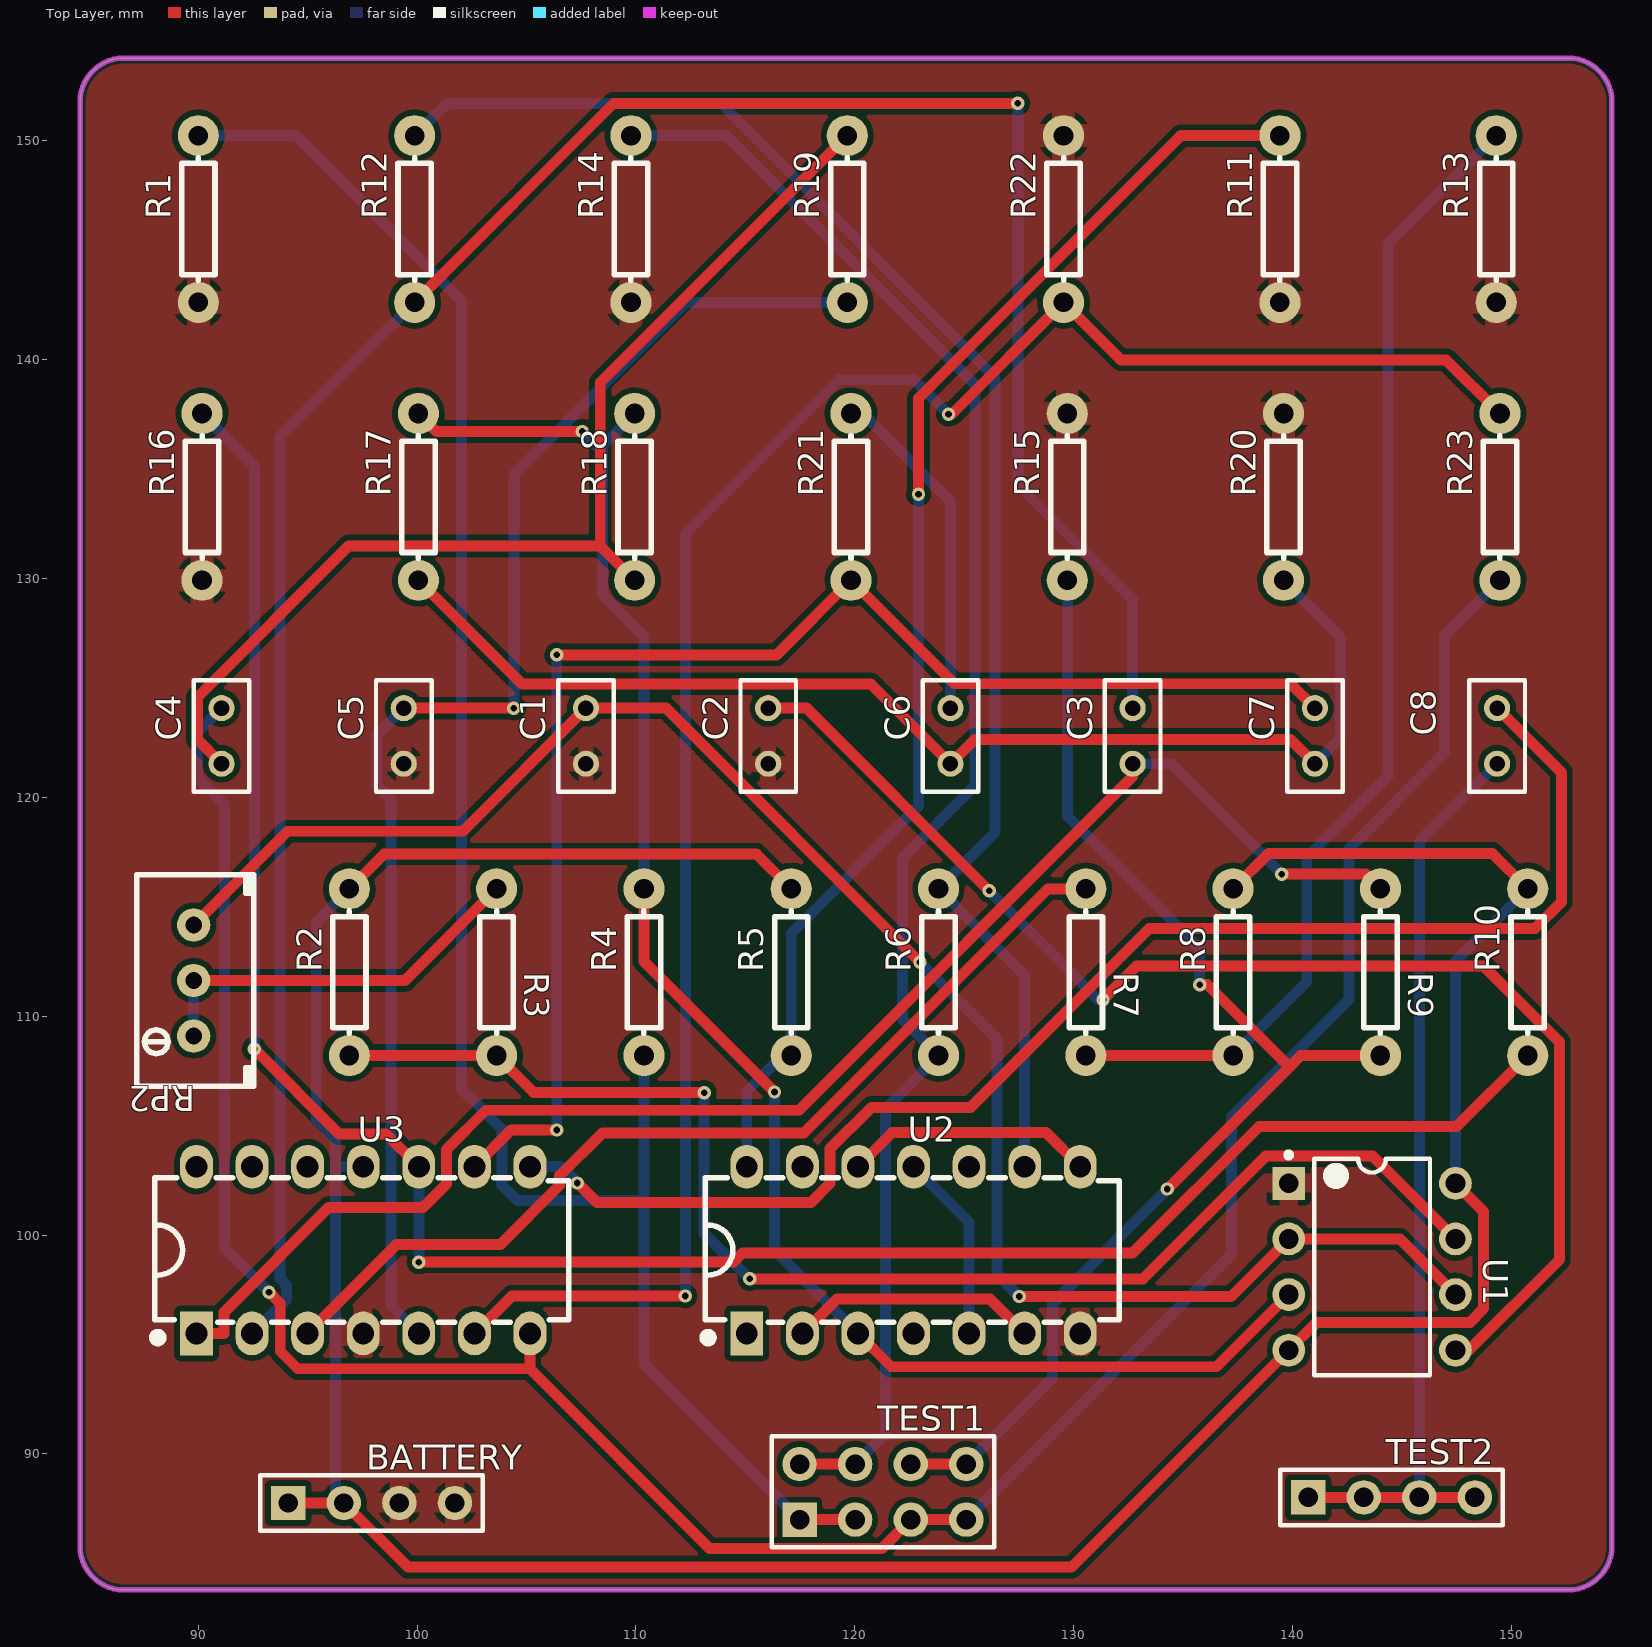
[diagram p0: Top Layer view]
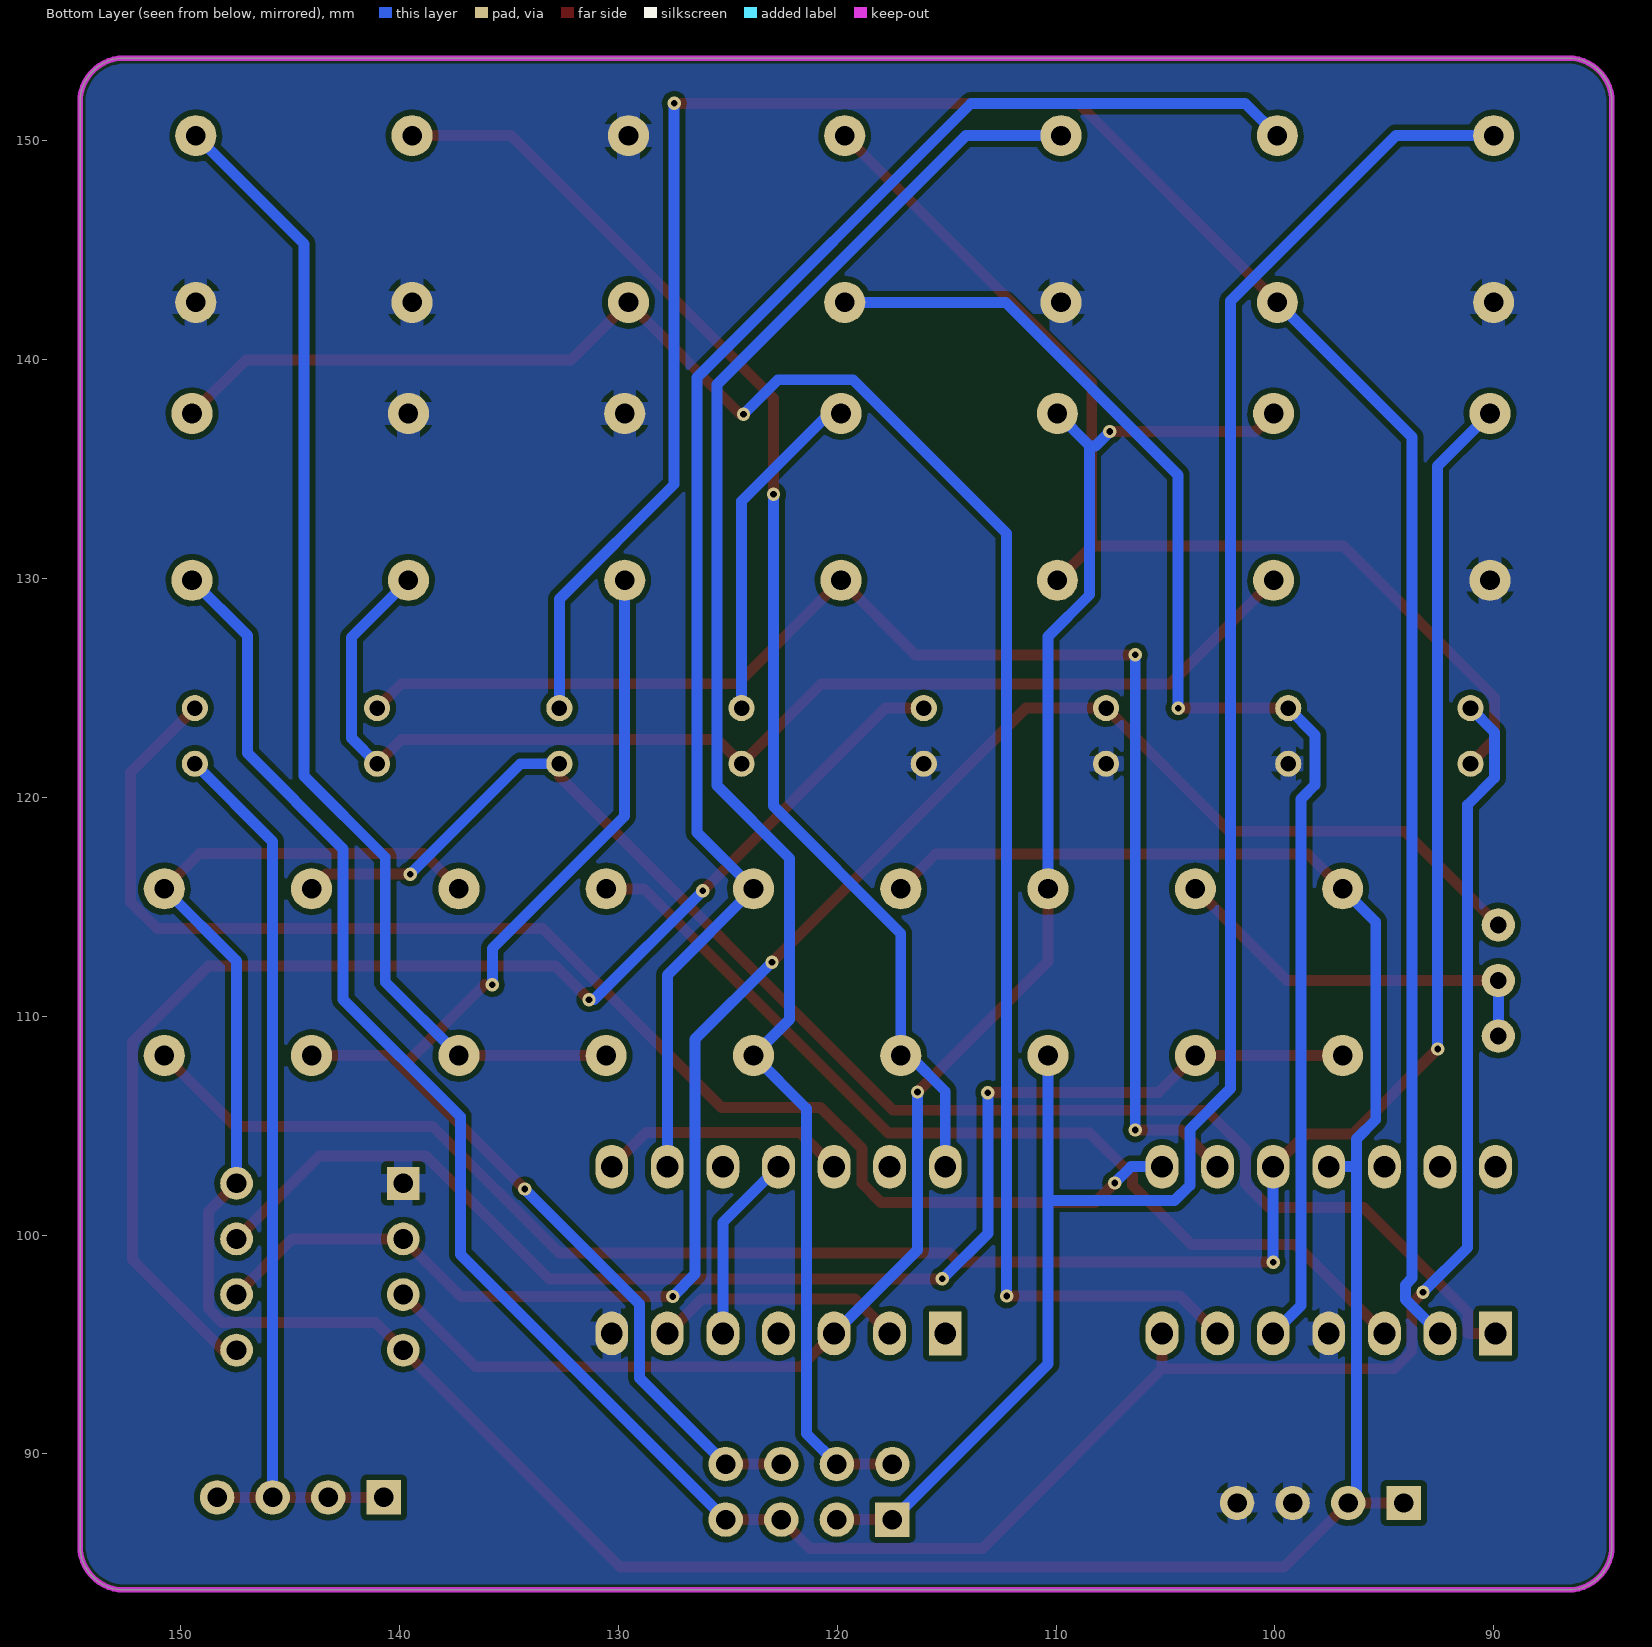
[diagram p1: Bottom Layer view, seen from below]
# Altium PCB MISC51938.pcbdoc
Units mm, origin at the board's own origin, x right, y up, seen from the top; angles counter-clockwise.
Board outline 70 x 70 mm, 2 copper layers (Top Layer, Bottom Layer), stack 0 mm thick; 38 components, 29 nets, 117 pads, 22 vias.

## Layer stack, top to bottom
Top Layer: signal copper (thickness not stored)
Bottom Layer: signal copper (thickness not stored)

## Board outline
84.597,151.785 cw(c86.597,151.785) 86.597,153.785 152.597,153.785 cw(c152.597,151.785) 154.597,151.785 154.597,85.785 cw(c152.597,85.785) 152.597,83.785 86.597,83.785 cw(c86.597,85.785) 84.597,85.785 84.597,151.785

## Design rules (kind name [scope] priority, off if disabled: settings)
BoardOutlineClearance Plane_Default_1 [All] p2 off: genericclearance=0.25 ignorepadtopadclearanceinfootprint=FALSE except(0: Arc-SplitContinuation Track-SplitContinuation SMDPad-SplitContinuation THPad-SplitContinuation Via-SplitContinuation Fill-SplitContinuation Region-SplitContinuation Poly-SplitContinuation Text-SplitContinuation Hole-SplitContinuation; 0.25: Arc-OutlineEdge Track-OutlineEdge SMDPad-OutlineEdge THPad-OutlineEdge Via-OutlineEdge Fill-OutlineEdge Region-OutlineEdge Poly-OutlineEdge Text-OutlineEdge Hole-OutlineEdge Arc-CutoutEdge Track-CutoutEdge SMDPad-CutoutEdge THPad-CutoutEdge Via-CutoutEdge Fill-CutoutEdge Region-CutoutEdge Poly-CutoutEdge Text-CutoutEdge Hole-CutoutEdge)
BoardOutlineClearance Copper_Default_1 [All] p4 off: genericclearance=0.25 ignorepadtopadclearanceinfootprint=FALSE except(0: Arc-SplitContinuation Track-SplitContinuation SMDPad-SplitContinuation THPad-SplitContinuation Via-SplitContinuation Fill-SplitContinuation Region-SplitContinuation Poly-SplitContinuation Text-SplitContinuation Hole-SplitContinuation; 0.25: Arc-OutlineEdge Track-OutlineEdge SMDPad-OutlineEdge THPad-OutlineEdge Via-OutlineEdge Fill-OutlineEdge Region-OutlineEdge Poly-OutlineEdge Text-OutlineEdge Hole-OutlineEdge Arc-CutoutEdge Track-CutoutEdge SMDPad-CutoutEdge THPad-CutoutEdge Via-CutoutEdge Fill-CutoutEdge Region-CutoutEdge Poly-CutoutEdge Text-CutoutEdge Hole-CutoutEdge)
BoardOutlineClearance Copper_gge9694_1 [All] p6 off: genericclearance=0.25 ignorepadtopadclearanceinfootprint=FALSE except(0: Arc-SplitContinuation Track-SplitContinuation SMDPad-SplitContinuation THPad-SplitContinuation Via-SplitContinuation Fill-SplitContinuation Region-SplitContinuation Poly-SplitContinuation Text-SplitContinuation Hole-SplitContinuation; 0.25: Arc-OutlineEdge Track-OutlineEdge SMDPad-OutlineEdge THPad-OutlineEdge Via-OutlineEdge Fill-OutlineEdge Region-OutlineEdge Text-OutlineEdge Hole-OutlineEdge Arc-CutoutEdge Track-CutoutEdge SMDPad-CutoutEdge THPad-CutoutEdge Via-CutoutEdge Fill-CutoutEdge Region-CutoutEdge Text-CutoutEdge Hole-CutoutEdge; 0.254: Poly-OutlineEdge Poly-CutoutEdge)
BoardOutlineClearance Copper_gge9712_1 [All] p8 off: genericclearance=0.25 ignorepadtopadclearanceinfootprint=FALSE except(0: Arc-SplitContinuation Track-SplitContinuation SMDPad-SplitContinuation THPad-SplitContinuation Via-SplitContinuation Fill-SplitContinuation Region-SplitContinuation Poly-SplitContinuation Text-SplitContinuation Hole-SplitContinuation; 0.25: Arc-OutlineEdge Track-OutlineEdge SMDPad-OutlineEdge THPad-OutlineEdge Via-OutlineEdge Fill-OutlineEdge Region-OutlineEdge Text-OutlineEdge Hole-OutlineEdge Arc-CutoutEdge Track-CutoutEdge SMDPad-CutoutEdge THPad-CutoutEdge Via-CutoutEdge Fill-CutoutEdge Region-CutoutEdge Text-CutoutEdge Hole-CutoutEdge; 0.254: Poly-OutlineEdge Poly-CutoutEdge)
BoardOutlineClearance Default_1 [All] p10: genericclearance=0.25 ignorepadtopadclearanceinfootprint=FALSE except(0: Arc-SplitContinuation Track-SplitContinuation SMDPad-SplitContinuation THPad-SplitContinuation Via-SplitContinuation Fill-SplitContinuation Region-SplitContinuation Poly-SplitContinuation Text-SplitContinuation Hole-SplitContinuation; 0.25: Arc-OutlineEdge Track-OutlineEdge SMDPad-OutlineEdge THPad-OutlineEdge Via-OutlineEdge Fill-OutlineEdge Region-OutlineEdge Poly-OutlineEdge Text-OutlineEdge Hole-OutlineEdge Arc-CutoutEdge Track-CutoutEdge SMDPad-CutoutEdge THPad-CutoutEdge Via-CutoutEdge Fill-CutoutEdge Region-CutoutEdge Poly-CutoutEdge Text-CutoutEdge Hole-CutoutEdge)
Clearance Plane_Default [All] p1 off: gap=0.25 ignorepadtopadclearanceinfootprint=FALSE
Clearance Copper_Default [All] p3 off: gap=0.25 ignorepadtopadclearanceinfootprint=FALSE
Clearance Copper_gge9694 [All] p5 off: gap=0.25 ignorepadtopadclearanceinfootprint=FALSE except(0.254: Poly-Track Poly-SMDPad Poly-THPad Poly-Via Poly-Fill Poly-Region Poly-Poly Poly-Arc Poly-Text Poly-Hole)
Clearance Copper_gge9712 [All] p7 off: gap=0.25 ignorepadtopadclearanceinfootprint=FALSE except(0.254: Poly-Track Poly-SMDPad Poly-THPad Poly-Via Poly-Fill Poly-Region Poly-Poly Poly-Arc Poly-Text Poly-Hole)
Clearance Default [All] p9: gap=0.25 ignorepadtopadclearanceinfootprint=FALSE
PasteMaskExpansion Common [All] p1: expansion=0
PlaneConnect Default_4 [All] p1: planeconnectstyle=Relief reliefexpansion=0.508 reliefentries=4 reliefconductorwidth=0 reliefairgap=0.254
PolygonConnect gge9694 [All] p1 off: connectstyle=Relief reliefconductorwidth=0 reliefentries=4 polygonreliefangle="90 Angle" airgapwidth=0.254 via.connectstyle=Relief via.reliefconductorwidth=0.254 via.reliefentries=4 via.polygonreliefangle="90 Angle" via.airgapwidth=0.254
PolygonConnect gge9712 [All] p2 off: connectstyle=Relief reliefconductorwidth=0 reliefentries=4 polygonreliefangle="90 Angle" airgapwidth=0.254 via.connectstyle=Relief via.reliefconductorwidth=0.254 via.reliefentries=4 via.polygonreliefangle="90 Angle" via.airgapwidth=0.254
PolygonConnect Default_5 [All] p3: connectstyle=Relief reliefconductorwidth=0 reliefentries=4 polygonreliefangle="90 Angle" airgapwidth=0.254 via.connectstyle=Relief via.reliefconductorwidth=0.254 via.reliefentries=4 via.polygonreliefangle="90 Angle" via.airgapwidth=0.254
RoutingVias Default_3 [All] p1: holewidth=0.305 width=0.61 viastyle="Through Hole" minholewidth=0.305 minwidth=0.61 maxholewidth=59.995 maxwidth=100.025
SolderMaskExpansion Common_1 [IsVia] p1: expansion=-25.4 istentingtop=TRUE
SolderMaskExpansion Common_1 [All] p2: expansion=0.051 istentingtop=FALSE
Width Default_2 [All] p1: maxlimit=25.4 minlimit=0.5 preferedwidth=0.5

## Components (designator, comment, footprint, x,y, rotation, side; value= is the part's Value field where it differs from the comment)
BATTERY "HDR-M-2.54_1x4" HDR-M-2.54_1X4 97.917,87.757 r0 top
C1 "1n" RAD-0.1 107.714,122.809 r90 top
C2 "0.01u" RAD-0.1 116.042,122.809 r90 top
C3 "10n" RAD-0.1 132.697,122.809 r90 top
C4 "1n" RAD-0.1 91.059,122.809 r90 top
C5 "1n" RAD-0.1 99.387,122.809 r90 top
C6 "0.1n" RAD-0.1 124.369,122.809 r90 top
C7 "0.1n" RAD-0.1 141.024,122.809 r90 top
C8 "1n" RAD-0.1 149.352,122.809 r90 top
R1 "60" R_AXIAL-0.3 90.001,146.431 r90 top
R2 "510" R_AXIAL-0.3 96.901,112.014 r90 top
R3 "12k" R_AXIAL-0.3 103.632,112.014 r270 top
R4 "540" R_AXIAL-0.3 110.363,112.014 r90 top
R5 "1k" R_AXIAL-0.3 117.094,112.014 r90 top
R6 "480" R_AXIAL-0.3 123.825,112.014 r90 top
R7 "1k" R_AXIAL-0.3 130.556,112.014 r270 top
R8 "300" R_AXIAL-0.3 137.287,112.014 r90 top
R9 "400" R_AXIAL-0.3 144.018,112.014 r270 top
R10 "1k" R_AXIAL-0.3 150.749,112.014 r90 top
R11 "1k" R_AXIAL-0.3 139.425,146.431 r90 top
R12 "1800" R_AXIAL-0.3 99.885,146.431 r90 top
R13 "100" R_AXIAL-0.3 149.31,146.431 r90 top
R14 "120" R_AXIAL-0.3 109.77,146.431 r90 top
R15 "200" R_AXIAL-0.3 129.709,133.731 r90 top
R16 "1350" R_AXIAL-0.3 90.17,133.731 r90 top
R17 "41k" R_AXIAL-0.3 100.055,133.731 r90 top
R18 "10k" R_AXIAL-0.3 109.94,133.731 r90 top
R19 "16500" R_AXIAL-0.3 119.655,146.431 r90 top
R20 "50" R_AXIAL-0.3 139.594,133.731 r90 top
R21 "90k" R_AXIAL-0.3 119.825,133.731 r90 top
R22 "3600" R_AXIAL-0.3 129.54,146.431 r90 top
R23 "720" R_AXIAL-0.3 149.479,133.731 r90 top
RP2 "R_3296W_US" RES-ADJ-TH_3296W 89.789,111.633 r180 top
TEST1 "test" HDR-M-2.54_2X4 121.285,88.265 r0 top
TEST2 "test" HDR-M-2.54_1X4 144.526,88.011 r0 top
U1 "100kHz" DIP-8_L9.8-W6.6-P2.54-LS7.6-BL 143.637,98.552 r270 top
U2 "SN74LS74N" DIP-14_L19.1-W6.4-P2.54-LS7.6-BL 122.682,99.314 r0 top
U3 "LM324_C5157701" DIP-14_L18.9-W6.4-P2.54-LS7.6-BL 97.536,99.314 r0 top

## Footprints (in the part's own frame and the unit in brackets; to place one, negate y for a bottom-side part, rotate by r counter-clockwise, add the part's x,y. Pads: shape width x height; smd on the part's side, far side on the other; paste and mask are expansions set on the pad)
DIP-8_L9.8-W6.6-P2.54-LS7.6-BL [mm]
  rect 1.5x1.5 hole 0.9: 1(-3.81,-3.81)
  round 1.5 hole 0.9: 2(-1.27,-3.81) 3(1.27,-3.81) 4(3.81,-3.81) 5(3.81,3.81) 6(1.27,3.81) 7(-1.27,3.81) 8(-3.81,3.81)
  silkscreen extent -5.23,-3.93 4.96,2.65
DIP-14_L18.9-W6.4-P2.54-LS7.6-BL [mm]
  rect 1.5x2 hole 1: 1(-7.62,-3.81)
  oval 1.5x2 hole 1: 2(-5.08,-3.81) 3(-2.54,-3.81) 4(0,-3.81) 5(2.54,-3.81) 6(5.08,-3.81) 7(7.62,-3.81) 8(7.62,3.81) 9(5.08,3.81) 10(2.54,3.81) 11(0,3.81) 12(-2.54,3.81) 13(-5.08,3.81) 14(-7.62,3.81)
  silkscreen extent -9.59,-4.2 9.4,3.3
DIP-14_L19.1-W6.4-P2.54-LS7.6-BL [mm]
  rect 1.5x2 hole 1: 1(-7.62,-3.81)
  oval 1.5x2 hole 1: 2(-5.08,-3.81) 3(-2.54,-3.81) 4(0,-3.81) 5(2.54,-3.81) 6(5.08,-3.81) 7(7.62,-3.81) 8(7.62,3.81) 9(5.08,3.81) 10(2.54,3.81) 11(0,3.81) 12(-2.54,3.81) 13(-5.08,3.81) 14(-7.62,3.81)
  silkscreen extent -9.59,-4.2 9.4,3.3
HDR-M-2.54_1X4 [mil]
  rect 62x62 hole 35: 1(-150,0)
  round 62 hole 35: 2(-50,0) 3(50,0) 4(150,0)
  silkscreen extent -200,-50 200,50
HDR-M-2.54_2X4 [mil]
  rect 62x62 hole 35: 1(-150,-50)
  round 62 hole 35: 2(-150,50) 3(-50,-50) 4(-50,50) 5(50,-50) 6(50,50) 7(150,-50) 8(150,50)
  silkscreen extent -200,-100 200,100
R_AXIAL-0.3 [mil]
  round 74 hole 35.4: 1(-150,0) 2(150,0)
  silkscreen extent -110,-30 110,30
RAD-0.1 [mil]
  round 47 hole 28: 1(-50,0) 2(50,0)
  silkscreen extent -100,-50 100,50
RES-ADJ-TH_3296W [mil]
  round 60 hole 30 copper offset -0.01,0.01: 1(0.01,99.99) 2(0.01,-0.01) 3(0.01,-100.01)
  silkscreen extent -108,-190 102,190

## Via types
v1: diameter 0.61, hole 0.305, Top Layer to Bottom Layer, 22 vias

## Nets (pads, with @x,y where several pads share a name; then routed paths per layer and width w, separated by ;. In a path a pad name is that pad's centre, name@x,y a point inside that pad or via, vN(x,y) a via of type N, cw(c..) or ccw(c..) an arc to the next point about the centre after c; other vN are vias at no path point)
C4_1: C4.1 R18.1 R19.2 | length 50.4
  Top Layer w0.5: C4.1 89.954,122.644 89.954,124.577 96.87,131.493 108.368,131.493 ; R18.1 108.368,131.493 ; R19.2 108.368,138.953 108.368,131.493
C5_2: C5.2 R19.1 U3.5 | length 64.1
  Top Layer w0.5: C5.2 v1(104.419,124.079)
  Bottom Layer w0.5: C5.2 98.161,122.853 98.161,120.577 98.806,119.931 98.806,96.774 U3.5 ; v1(104.419,124.079) 104.419,134.741 112.299,142.621 R19.1
C6_1: C6.1 C7.1 R17.1 R20.1 | length 55.3
  Top Layer w0.5: R17.1 104.798,125.178 120.731,125.178 C6.1 125.482,122.651 139.912,122.651 C7.1
  Bottom Layer w0.5: R20.1 142.199,127.316 142.199,122.713 C7.1
C6_2: C6.2 R21.2 | length 15.7
  Bottom Layer w0.5: R21.2 120.363,137.541 124.369,133.534 C6.2
C7_2: C7.2 R21.1 U3.9 | length 64.6
  Top Layer w0.5: U3.9 104.296,104.804 v1(106.378,104.804) ; v1(106.378,126.515) 116.418,126.515 R21.1 124.552,125.194 139.91,125.194 C7.2
  Bottom Layer w0.5: v1(106.378,104.804) v1(106.378,126.515)
C8_1: C8.1 TEST2.1 TEST2.2 TEST2.3 TEST2.4 | length 42.6
  Top Layer w0.5: TEST2.1 TEST2.2 TEST2.3 TEST2.4
  Bottom Layer w0.5: TEST2.3 145.796,117.983 C8.1
GND: BATTERY.3 BATTERY.4 C1.1 C2.1 C5.1 R1.1 R11.1 R13.1 R14.1 R15.2 R16.1 R20.2 R22.2 U1.1 U2.7 U3.4
R3_1: R3.1 RP2.1 RP2.2 | length 18.1
  Top Layer w0.5: RP2.2 99.441,111.633 R3.1
  Bottom Layer w0.5: RP2.1 RP2.2
R4_1: R1.2 R4.1 TEST1.1 TEST1.3 | length 89.8
  Top Layer w0.5: TEST1.1 TEST1.3
  Bottom Layer w0.5: R1.2 94.461,150.241 102.021,142.681 102.021,106.696 103.887,104.83 103.887,102.263 104.579,101.572 110.363,101.572 ; R4.1 110.363,101.572 ; TEST1.1 110.363,94.107 110.363,101.572
R7_1: R7.1 U3.3 | length 44.2
  Top Layer w0.5: U3.3 99.062,99.569 103.804,99.569 106.512,102.277 106.512,102.712 108.469,104.669 117.665,104.669 128.82,115.824 R7.1
R7_2: R7.2 R8.1 R13.2 | length 53.7
  Top Layer w0.5: R7.2 R8.1
  Bottom Layer w0.5: R8.1 140.653,111.57 140.653,117.266 144.368,120.98 144.368,145.299 R13.2
R10_1: R10.1 R16.2 U3.10 | length 98.7
  Top Layer w0.5: v1(92.558,108.504) 96.437,104.626 98.574,104.626 U3.10 ; v1(100.076,98.763) 114.447,98.763 114.858,99.174 132.694,99.174 138.479,104.958 147.503,104.958 R10.1
  Bottom Layer w0.5: R16.2 92.558,135.153 v1(92.558,108.504) ; v1(100.076,98.763) U3.10
TEST1_2: R6.1 R14.2 TEST1.2 TEST1.4 | length 75.9
  Top Layer w0.5: TEST1.2 TEST1.4
  Bottom Layer w0.5: R14.2 114.117,150.241 125.496,138.862 125.496,120.542 122.172,117.218 122.172,109.857 R6.1 121.412,105.791 121.412,90.932 TEST1.4
TEST1_5: C4.2 R23.1 TEST1.5 TEST1.7 U3.7 | length 121.7
  Top Layer w0.5: v1(93.228,97.39) 93.744,96.874 93.744,94.691 94.544,93.891 105.156,93.891 ; U3.7 105.156,93.891 ; TEST1.7 TEST1.5 121.242,85.682 113.366,85.682 105.156,93.891
  Bottom Layer w0.5: C4.2 89.956,122.976 89.956,120.896 91.186,119.665 91.186,99.432 v1(93.228,97.39) ; TEST1.7 137.22,99.12 137.22,105.407 142.576,110.764 142.576,117.649 146.952,122.025 146.952,127.394 R23.1
TEST1_6: R9.2 R15.1 TEST1.6 TEST1.8 | length 57.8
  Top Layer w0.5: TEST1.6 TEST1.8 ; v1(134.282,102.108) 139.861,107.687 ; v1(135.758,111.442) 136.106,111.442 139.861,107.687 ; R9.2 140.378,108.204 139.861,107.687
  Bottom Layer w0.5: TEST1.8 129.032,93.472 129.032,96.858 v1(134.282,102.108) ; R15.1 129.709,119.154 135.758,113.105 v1(135.758,111.442)
U1_2: C1.2 RP2.3 U1.2 U1.6 | length 81.3
  Top Layer w0.5: RP2.3 94.07,118.455 102.09,118.455 C1.2 111.369,124.079 v1(122.979,112.469) ; v1(127.51,97.195) 137.2,97.195 U1.2 144.907,99.822 U1.6
  Bottom Layer w0.5: v1(122.979,112.469) 126.492,108.956 126.492,98.213 v1(127.51,97.195)
U1_3: R4.2 R17.2 R18.2 U1.3 U2.3 | length 78.2
  Top Layer w0.5: R17.2 100.874,136.722 v1(107.54,136.722) ; R4.2 110.363,112.51 v1(116.332,106.541) ; U2.3 121.664,93.982 136.527,93.982 U1.3
  Bottom Layer w0.5: v1(107.54,136.722) 108.201,136.062 108.46,136.062 ; R18.2 108.46,136.062 ; R4.2 110.363,127.36 108.46,129.263 108.46,136.062 ; v1(116.332,106.541) 116.332,99.314 U2.3
U1_5: C2.2 U1.5 | length 60.2
  Top Layer w0.5: C2.2 117.796,124.079 v1(126.146,115.729) ; v1(131.343,110.76) 132.877,112.294 148.725,112.294 152.195,108.825 152.195,98.875 148.062,94.742 U1.5
  Bottom Layer w0.5: v1(126.146,115.729) 131.115,110.76 v1(131.343,110.76)
U1_7: R2.1 R3.2 U1.7 | length 62.4
  Top Layer w0.5: R2.1 R3.2 105.326,106.51 v1(113.114,106.51) ; v1(115.192,98.002) 133.171,98.002 138.784,103.614 143.655,103.614 U1.7
  Bottom Layer w0.5: v1(113.114,106.51) 113.114,100.08 v1(115.192,98.002)
U2_2: U2.2 U2.6 | length 11.5
  Top Layer w0.5: U2.2 119.178,97.08 126.186,97.08 U2.6
U2_5: U2.5 U2.11 | length 8.7
  Bottom Layer w0.5: U2.11 125.222,100.584 U2.5
U2_8: U2.8 U2.12 | length 11.5
  Top Layer w0.5: U2.12 121.708,104.69 128.736,104.69 U2.8
U2_9: R6.2 R12.2 U2.9 | length 71.1
  Bottom Layer w0.5: R12.2 101.363,151.719 113.876,151.719 126.405,139.19 126.405,118.404 R6.2 127.762,111.887 U2.9
U2_14: R5.1 R11.2 U2.14 | length 60.1
  Top Layer w0.5: v1(122.911,133.851) 122.911,138.241 134.912,150.241 R11.2
  Bottom Layer w0.5: U2.14 115.062,106.57 116.696,108.204 R5.1 117.094,113.785 122.911,119.602 v1(122.911,133.851)
U3_1: C3.1 R9.1 U3.1 | length 69.1
  Top Layer w0.5: U3.1 91.167,95.504 91.167,96.469 95.957,101.259 100.268,101.259 101.346,102.337 101.346,103.913 103.136,105.703 117.442,105.703 132.697,120.958 C3.1 ; v1(139.51,116.495) 143.347,116.495 R9.1
  Bottom Layer w0.5: C3.1 134.465,121.539 v1(139.51,116.495)
U3_2: C3.2 R12.1 U3.2 | length 111.6
  Top Layer w0.5: R12.1 108.984,151.719 v1(127.447,151.719)
  Bottom Layer w0.5: U3.2 92.483,95.504 94.035,97.056 94.035,97.724 93.726,98.033 93.726,136.461 R12.1 ; v1(127.447,151.719) 127.447,134.309 132.697,129.059 C3.2
U3_6: R22.1 R23.2 U3.6 | length 90.2
  Top Layer w0.5: U3.6 104.33,97.217 v1(112.254,97.217) ; v1(124.281,137.509) 124.428,137.509 R22.1 132.165,139.996 147.024,139.996 R23.2
  Bottom Layer w0.5: v1(112.254,97.217) 112.254,132.069 119.271,139.086 122.705,139.086 v1(124.281,137.509)
U3_8: C8.2 U3.8 | length 64.5
  Top Layer w0.5: v1(107.319,102.378) 108.21,101.487 117.991,101.487 118.872,102.368 118.872,103.948 120.761,105.837 125.279,105.837 133.453,114.011 151.073,114.011 152.287,115.225 152.287,121.144 C8.2
  Bottom Layer w0.5: U3.8 106.573,103.124 v1(107.319,102.378)
VCC: BATTERY.1 BATTERY.2 R2.2 R5.2 R8.2 R10.2 U1.4 U1.8 U3.11 | length 148.6
  Top Layer w0.5: BATTERY.1 95.395,87.757 BATTERY.2 99.578,84.826 129.911,84.826 U1.4 141.097,96.012 148.111,96.012 148.735,96.636 148.735,101.074 U1.8 ; R2.2 98.497,117.42 115.498,117.42 R5.2 ; R8.2 138.905,117.442 149.131,117.442 R10.2
  Bottom Layer w0.5: BATTERY.2 96.266,88.138 96.266,103.124 ; R2.2 95.39,114.313 95.39,105.27 96.266,104.394 96.266,103.124 ; U3.11 96.266,103.124 ; U1.8 147.447,112.522 R10.2
pads on no net: U2.1 U2.4 U2.10 U2.13 U3.12 U3.13 U3.14

## Polygon pours and split planes (outlines as drawn)
GND on Top Layer (solid, remove dead copper, pour order 2): 80.772,156.845 80.772,82.677 83.312,80.137 158.623,80.137 159.766,81.28 159.766,157.353 158.75,158.369
GND on Bottom Layer (solid, remove dead copper, pour order 6): 76.2,159.512 76.2,78.486 78.486,76.2 160.909,76.2 164.084,79.375 164.084,158.496 161.544,161.036

## Keep-outs
Board Outline Layer:
  the board outline again, w0.254